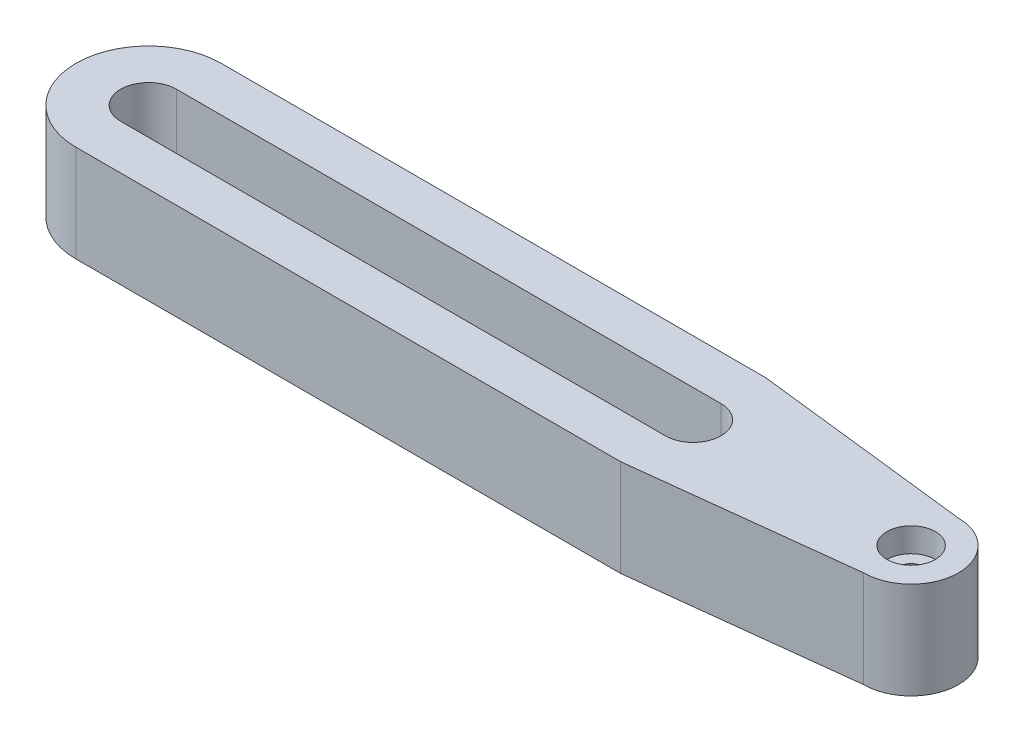
from build123d import *

# Parameters (mm, degrees)
BOSS_EXTRUDE1_DEPTH = 8
SKETCH2_R           = 2
CUT_EXTRUDE1_DEPTH  = 2
SKETCH3_R           = 1
CUT_EXTRUDE2_DEPTH  = 68.657428272


with BuildPart() as part:
    # Sketch1 → Boss-Extrude1 (new body)
    with BuildSketch(Plane(origin=(0, 0, 0), x_dir=(1, 0, 0), z_dir=(0, 1, 0))):
        with BuildLine():
            Line((0, 6), (45, 6))
            Line((45, 6), (63, 3.914330307))
            ThreePointArc((63, 3.914330307), (66.914330307, 0), (63, -3.914330307))
            Line((63, -3.914330307), (45, -6))
            Line((45, -6), (0, -6))
            ThreePointArc((0, -6), (-6, 0), (0, 6))
        make_face()
        with BuildLine():
            Line((0, 2.3), (45, 2.3))
            ThreePointArc((45, 2.3), (47.3, 0), (45, -2.3))
            Line((45, -2.3), (0, -2.3))
            ThreePointArc((0, -2.3), (-2.3, 0), (0, 2.3))
        make_face(mode=Mode.SUBTRACT)
    extrude(amount=BOSS_EXTRUDE1_DEPTH)

    # Sketch2 → Cut-Extrude1 (cut)
    with BuildSketch(Plane(origin=(0, 8, 0), x_dir=(1, 0, 0), z_dir=(0, 1, 0))):
        with Locations(Location((63, 0, 0), (0, 0, 270))):
            Circle(SKETCH2_R)
    extrude(amount=-CUT_EXTRUDE1_DEPTH, mode=Mode.SUBTRACT)

    # Sketch3 → Cut-Extrude2 (cut, through all)
    with BuildSketch(Plane.XZ):
        with Locations(Location((63, 0, 0), (0, 0, 270))):
            Circle(SKETCH3_R)
    extrude(amount=-CUT_EXTRUDE2_DEPTH, mode=Mode.SUBTRACT)


solid = part.part
